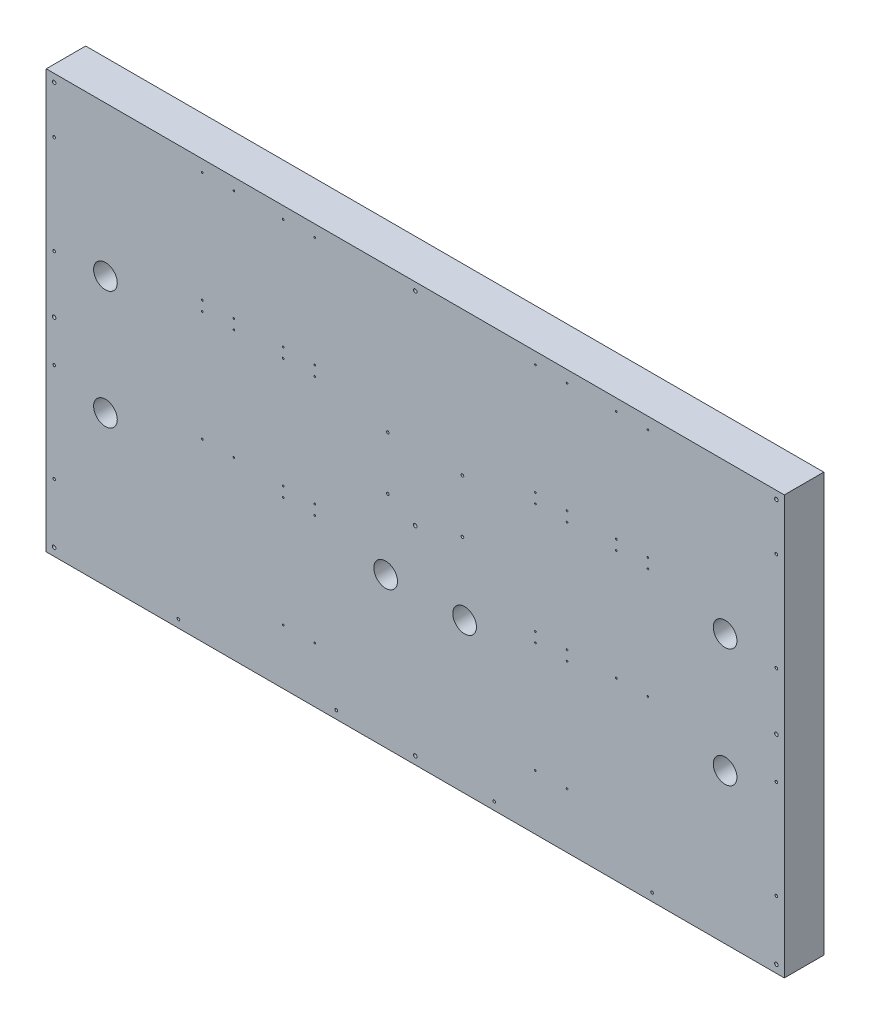
from build123d import *

# Parameters (mm, degrees)
SKETCH_1_W                           = 1870
SKETCH_1_H                           = 1060
EXTRUDE_1_DEPTH                      = 50
HOLE_WIZARD_M8_1_D                   = 6.8
PATTERN_LINEAR_1_COUNT               = 2
PATTERN_LINEAR_1_PITCH               = 135
PATTERN_LINEAR_1_COUNT_DIR2          = 2
PATTERN_LINEAR_1_PITCH_DIR2          = 189
HOLE_WIZARD_2_D                      = 9
HOLE_WIZARD_2_CBORE_D                = 15
HOLE_WIZARD_2_CBORE_DEPTH            = 50
PATTERN_LINEAR_2_COUNT               = 2
PATTERN_LINEAR_2_PITCH               = 515
PATTERN_LINEAR_3_COUNT               = 2
PATTERN_LINEAR_3_PITCH               = 915
PATTERN_LINEAR_3_COPY_1_D            = 9
PATTERN_LINEAR_3_COPY_1_CBORE_D      = 15
PATTERN_LINEAR_3_COPY_1_CBORE_DEPTH  = 50
HOLE_WIZARD_M5_1_D                   = 4.2
PATTERN_LINEAR_5_COUNT               = 2
PATTERN_LINEAR_5_PITCH               = 280
PATTERN_LINEAR_6_COUNT               = 2
PATTERN_LINEAR_6_PITCH               = 305
PATTERN_LINEAR_6_COPY_1_D            = 4.2
PATTERN_LINEAR_7_COUNT               = 2
PATTERN_LINEAR_7_PITCH               = 205
PATTERN_LINEAR_7_COPY_1_D            = 4.2
PATTERN_LINEAR_7_COPY_2_D            = 4.2
PATTERN_LINEAR_7_COPY_3_D            = 4.2
PATTERN_LINEAR_8_COUNT               = 2
PATTERN_LINEAR_8_PITCH               = 844
PATTERN_LINEAR_8_COPY_1_D            = 4.2
PATTERN_LINEAR_8_COPY_2_D            = 4.2
PATTERN_LINEAR_8_COPY_3_D            = 4.2
PATTERN_LINEAR_8_COPY_4_D            = 4.2
PATTERN_LINEAR_8_COPY_5_D            = 4.2
PATTERN_LINEAR_8_COPY_6_D            = 4.2
PATTERN_LINEAR_8_COPY_7_D            = 4.2
SKETCH_10_R                          = 2.1
CUT_EXTRUDE_1_DEPTH                  = 1080.409560825
PATTERN_LINEAR_9_COUNT               = 2
PATTERN_LINEAR_9_PITCH               = 639
SKETCH_12_R                          = 30
CUT_EXTRUDE_2_DEPTH                  = 1080.409560825
MIRROR_2_COPY_1_D                    = 9
MIRROR_2_COPY_1_CBORE_D              = 15
MIRROR_2_COPY_1_CBORE_DEPTH          = 50
SKETCH_13_R                          = 30
CUT_EXTRUDE_3_DEPTH                  = 1080.409560825
HOLE_WIZARD_M8_2_D                   = 6.8
PATTERN_LINEAR_10_COUNT              = 4
PATTERN_LINEAR_10_PITCH              = 250
MIRROR_3_COPY_1_D                    = 6.8
MIRROR_3_COPY_2_D                    = 6.8
MIRROR_3_COPY_3_D                    = 6.8
HOLE_WIZARD_M8_3_D                   = 6.8
PATTERN_LINEAR_11_COUNT              = 4
PATTERN_LINEAR_11_PITCH              = 400
PATTERN_LINEAR_12_COUNT              = 2
PATTERN_LINEAR_12_PITCH              = 1020
PATTERN_LINEAR_13_COPY_1_D           = 9
PATTERN_LINEAR_13_COPY_1_CBORE_D     = 15
PATTERN_LINEAR_13_COPY_1_CBORE_DEPTH = 50
PATTERN_LINEAR_13_COPY_2_D           = 9
PATTERN_LINEAR_13_COPY_2_CBORE_D     = 15
PATTERN_LINEAR_13_COPY_2_CBORE_DEPTH = 50
MIRROR_4_COPY_1_D                    = 9
MIRROR_4_COPY_1_CBORE_D              = 15
MIRROR_4_COPY_1_CBORE_DEPTH          = 50
MIRROR_4_COPY_2_D                    = 9
MIRROR_4_COPY_2_CBORE_D              = 15
MIRROR_4_COPY_2_CBORE_DEPTH          = 50


with BuildPart() as part:
    # 草图1 → 凸台-拉伸1 (new, symmetric)
    with BuildSketch(Plane.XY):
        Rectangle(SKETCH_1_W, SKETCH_1_H)
    extrude(amount=EXTRUDE_1_DEPTH, both=True)

    # M8 螺纹孔1 (through all)
    with Locations(Plane.XY.offset(50)):
        with Locations((-69.5, 30)):
            hole_wizard_m8_1 = Hole(HOLE_WIZARD_M8_1_D / 2)

    # 阵列(线性)1: Hole Wizard M8 _1 2 × 2
    with Locations(*[(j * PATTERN_LINEAR_1_PITCH_DIR2, i * PATTERN_LINEAR_1_PITCH, 0) for i in range(PATTERN_LINEAR_1_COUNT) for j in range(PATTERN_LINEAR_1_COUNT_DIR2) if (i, j) != (0, 0)]):
        add(hole_wizard_m8_1, mode=Mode.SUBTRACT)

    # 打孔尺寸(%根据)内六角圆柱头螺钉的类型2 (through all)
    with Locations(Plane(origin=(0, 0, -50), x_dir=(-1, 0, 0), z_dir=(0, 0, -1))):
        with Locations((-915, 510)):
            hole_wizard_2 = CounterBoreHole(HOLE_WIZARD_2_D / 2, HOLE_WIZARD_2_CBORE_D / 2, HOLE_WIZARD_2_CBORE_DEPTH)

    # 阵列(线性)2: 打孔尺寸(%根据)内六角圆柱头螺钉的类型2 ×2
    with Locations(*[(0, -i * PATTERN_LINEAR_2_PITCH, 0) for i in range(1, PATTERN_LINEAR_2_COUNT)]):
        add(hole_wizard_2, mode=Mode.SUBTRACT)

    # 阵列(线性)3: 打孔尺寸(%根据)内六角圆柱头螺钉的类型2 ×2
    with Locations(*[(-i * PATTERN_LINEAR_3_PITCH, 0, 0) for i in range(1, PATTERN_LINEAR_3_COUNT)]):
        add(hole_wizard_2, mode=Mode.SUBTRACT)

    # 阵列(线性)3 copy 1 (through all)
    with Locations(Plane(origin=(-915, -515, -50), x_dir=(-1, 0, 0), z_dir=(0, 0, -1))):
        with Locations((-915, 510)):
            CounterBoreHole(PATTERN_LINEAR_3_COPY_1_D / 2, PATTERN_LINEAR_3_COPY_1_CBORE_D / 2, PATTERN_LINEAR_3_COPY_1_CBORE_DEPTH)

    # M5 螺纹孔1 (through all)
    with Locations(Plane(origin=(0, 0, -50), x_dir=(-1, 0, 0), z_dir=(0, 0, -1))):
        with Locations((-589.5, 500), (-509.5, 500)):
            hole_wizard_m5_1 = Hole(HOLE_WIZARD_M5_1_D / 2)

    # 阵列(线性)5: M5 螺纹孔1 ×2
    with Locations(*[(0, -i * PATTERN_LINEAR_5_PITCH, 0) for i in range(1, PATTERN_LINEAR_5_COUNT)]):
        add(hole_wizard_m5_1, mode=Mode.SUBTRACT)

    # 阵列(线性)6: M5 螺纹孔1 ×2
    with Locations(*[(0, -i * PATTERN_LINEAR_6_PITCH, 0) for i in range(1, PATTERN_LINEAR_6_COUNT)]):
        add(hole_wizard_m5_1, mode=Mode.SUBTRACT)

    # 阵列(线性)6 copy 1 (through all)
    with Locations(Plane(origin=(0, -585, -50), x_dir=(-1, 0, 0), z_dir=(0, 0, -1))):
        with Locations((-589.5, 500), (-509.5, 500)):
            Hole(PATTERN_LINEAR_6_COPY_1_D / 2)

    # 阵列(线性)7: M5 螺纹孔1 ×2
    with Locations(*[(-i * PATTERN_LINEAR_7_PITCH, 0, 0) for i in range(1, PATTERN_LINEAR_7_COUNT)]):
        add(hole_wizard_m5_1, mode=Mode.SUBTRACT)

    # 阵列(线性)7 copy 1 (through all)
    with Locations(Plane(origin=(-205, -280, -50), x_dir=(-1, 0, 0), z_dir=(0, 0, -1))):
        with Locations((-589.5, 500), (-509.5, 500)):
            Hole(PATTERN_LINEAR_7_COPY_1_D / 2)

    # 阵列(线性)7 copy 2 (through all)
    with Locations(Plane(origin=(-205, -305, -50), x_dir=(-1, 0, 0), z_dir=(0, 0, -1))):
        with Locations((-589.5, 500), (-509.5, 500)):
            Hole(PATTERN_LINEAR_7_COPY_2_D / 2)

    # 阵列(线性)7 copy 3 (through all)
    with Locations(Plane(origin=(-205, -585, -50), x_dir=(-1, 0, 0), z_dir=(0, 0, -1))):
        with Locations((-589.5, 500), (-509.5, 500)):
            Hole(PATTERN_LINEAR_7_COPY_3_D / 2)

    # 阵列(线性)8: M5 螺纹孔1 ×2
    with Locations(*[(-i * PATTERN_LINEAR_8_PITCH, 0, 0) for i in range(1, PATTERN_LINEAR_8_COUNT)]):
        add(hole_wizard_m5_1, mode=Mode.SUBTRACT)

    # 阵列(线性)8 copy 1 (through all)
    with Locations(Plane(origin=(-844, -280, -50), x_dir=(-1, 0, 0), z_dir=(0, 0, -1))):
        with Locations((-589.5, 500), (-509.5, 500)):
            Hole(PATTERN_LINEAR_8_COPY_1_D / 2)

    # 阵列(线性)8 copy 2 (through all)
    with Locations(Plane(origin=(-844, -305, -50), x_dir=(-1, 0, 0), z_dir=(0, 0, -1))):
        with Locations((-589.5, 500), (-509.5, 500)):
            Hole(PATTERN_LINEAR_8_COPY_2_D / 2)

    # 阵列(线性)8 copy 3 (through all)
    with Locations(Plane(origin=(-844, -585, -50), x_dir=(-1, 0, 0), z_dir=(0, 0, -1))):
        with Locations((-589.5, 500), (-509.5, 500)):
            Hole(PATTERN_LINEAR_8_COPY_3_D / 2)

    # 阵列(线性)8 copy 4 (through all)
    with Locations(Plane(origin=(-1049, 0, -50), x_dir=(-1, 0, 0), z_dir=(0, 0, -1))):
        with Locations((-589.5, 500), (-509.5, 500)):
            Hole(PATTERN_LINEAR_8_COPY_4_D / 2)

    # 阵列(线性)8 copy 5 (through all)
    with Locations(Plane(origin=(-1049, -280, -50), x_dir=(-1, 0, 0), z_dir=(0, 0, -1))):
        with Locations((-589.5, 500), (-509.5, 500)):
            Hole(PATTERN_LINEAR_8_COPY_5_D / 2)

    # 阵列(线性)8 copy 6 (through all)
    with Locations(Plane(origin=(-1049, -305, -50), x_dir=(-1, 0, 0), z_dir=(0, 0, -1))):
        with Locations((-589.5, 500), (-509.5, 500)):
            Hole(PATTERN_LINEAR_8_COPY_6_D / 2)

    # 阵列(线性)8 copy 7 (through all)
    with Locations(Plane(origin=(-1049, -585, -50), x_dir=(-1, 0, 0), z_dir=(0, 0, -1))):
        with Locations((-589.5, 500), (-509.5, 500)):
            Hole(PATTERN_LINEAR_8_COPY_7_D / 2)

    # 草图10 → 切除-拉伸1 (cut, through all)
    with BuildSketch(Plane(origin=(0, 0, -50), x_dir=(-1, 0, 0), z_dir=(0, 0, -1))):
        with Locations((-304.5, -390)):
            Circle(SKETCH_10_R)
        with Locations((-384.5, -390)):
            Circle(SKETCH_10_R)
        with Locations((-304.5, -110)):
            Circle(SKETCH_10_R)
        with Locations((-384.5, -110)):
            Circle(SKETCH_10_R)
    cut_extrude_1 = extrude(amount=-CUT_EXTRUDE_1_DEPTH, mode=Mode.SUBTRACT)

    # 阵列(线性)9: 切除-拉伸1 ×2
    with Locations(*[(-i * PATTERN_LINEAR_9_PITCH, 0, 0) for i in range(1, PATTERN_LINEAR_9_COUNT)]):
        add(cut_extrude_1, mode=Mode.SUBTRACT)

    # 草图12 → 切除-拉伸2 (cut, through all)
    with BuildSketch(Plane(origin=(0, 0, -50), x_dir=(-1, 0, 0), z_dir=(0, 0, -1))):
        with Locations((-785, 150)):
            Circle(SKETCH_12_R)
        with Locations((-785, -150)):
            Circle(SKETCH_12_R)
    cut_extrude_2 = extrude(amount=-CUT_EXTRUDE_2_DEPTH, mode=Mode.SUBTRACT)

    # 镜向1: 切除-拉伸2 across plane
    add(cut_extrude_2.mirror(Plane(origin=(0, 0, 0), x_dir=(0, 0, 1), z_dir=(1, 0, 0))), mode=Mode.SUBTRACT)

    # 镜向2: 打孔尺寸(%根据)内六角圆柱头螺钉的类型2 across plane
    add(hole_wizard_2.mirror(Plane(origin=(0, 0, 0), x_dir=(0, 0, 1), z_dir=(1, 0, 0))), mode=Mode.SUBTRACT)

    # 镜向2 copy 1 (through all)
    with Locations(Plane(origin=(0, -515, -50), x_dir=(1, 0, 0), z_dir=(0, 0, -1))):
        with Locations((-915, -510)):
            CounterBoreHole(MIRROR_2_COPY_1_D / 2, MIRROR_2_COPY_1_CBORE_D / 2, MIRROR_2_COPY_1_CBORE_DEPTH)

    # 草图13 → 切除-拉伸3 (cut, through all)
    with BuildSketch(Plane(origin=(0, 0, -50), x_dir=(-1, 0, 0), z_dir=(0, 0, -1))):
        with Locations((-125, -150)):
            Circle(SKETCH_13_R)
        with Locations((75, -150)):
            Circle(SKETCH_13_R)
    extrude(amount=-CUT_EXTRUDE_3_DEPTH, mode=Mode.SUBTRACT)

    # M8 螺纹孔2 (through all)
    with Locations(Plane(origin=(0, 0, -50), x_dir=(-1, 0, 0), z_dir=(0, 0, -1))):
        with Locations((-915, 390)):
            hole_wizard_m8_2 = Hole(HOLE_WIZARD_M8_2_D / 2)

    # 阵列(线性)10: M8 螺纹孔2 ×4
    with Locations(*[(0, -i * PATTERN_LINEAR_10_PITCH, 0) for i in range(1, PATTERN_LINEAR_10_COUNT)]):
        add(hole_wizard_m8_2, mode=Mode.SUBTRACT)

    # 镜向3: M8 螺纹孔2 across plane
    add(hole_wizard_m8_2.mirror(Plane(origin=(0, 0, 0), x_dir=(0, 0, 1), z_dir=(1, 0, 0))), mode=Mode.SUBTRACT)

    # 镜向3 copy 1 (through all)
    with Locations(Plane(origin=(0, -250, -50), x_dir=(1, 0, 0), z_dir=(0, 0, -1))):
        with Locations((-915, -390)):
            Hole(MIRROR_3_COPY_1_D / 2)

    # 镜向3 copy 2 (through all)
    with Locations(Plane(origin=(0, -500, -50), x_dir=(1, 0, 0), z_dir=(0, 0, -1))):
        with Locations((-915, -390)):
            Hole(MIRROR_3_COPY_2_D / 2)

    # 镜向3 copy 3 (through all)
    with Locations(Plane(origin=(0, -750, -50), x_dir=(1, 0, 0), z_dir=(0, 0, -1))):
        with Locations((-915, -390)):
            Hole(MIRROR_3_COPY_3_D / 2)

    # M8 螺纹孔3 (through all)
    with Locations(Plane(origin=(0, 0, -50), x_dir=(-1, 0, 0), z_dir=(0, 0, -1))):
        with Locations((-600, -510)):
            hole_wizard_m8_3 = Hole(HOLE_WIZARD_M8_3_D / 2)

    # 阵列(线性)11: M8 螺纹孔3 ×4
    with Locations(*[(-i * PATTERN_LINEAR_11_PITCH, 0, 0) for i in range(1, PATTERN_LINEAR_11_COUNT)]):
        add(hole_wizard_m8_3, mode=Mode.SUBTRACT)

    # 阵列(线性)12: 打孔尺寸(%根据)内六角圆柱头螺钉的类型2 ×2
    with Locations(*[(0, -i * PATTERN_LINEAR_12_PITCH, 0) for i in range(1, PATTERN_LINEAR_12_COUNT)]):
        add(hole_wizard_2, mode=Mode.SUBTRACT)

    # 阵列(线性)13 copy 1 (through all)
    with Locations(Plane(origin=(-915, -1020, -50), x_dir=(-1, 0, 0), z_dir=(0, 0, -1))):
        with Locations((-915, 510)):
            CounterBoreHole(PATTERN_LINEAR_13_COPY_1_D / 2, PATTERN_LINEAR_13_COPY_1_CBORE_D / 2, PATTERN_LINEAR_13_COPY_1_CBORE_DEPTH)

    # 阵列(线性)13 copy 2 (through all)
    with Locations(Plane(origin=(-915, 0, -50), x_dir=(-1, 0, 0), z_dir=(0, 0, -1))):
        with Locations((-915, 510)):
            CounterBoreHole(PATTERN_LINEAR_13_COPY_2_D / 2, PATTERN_LINEAR_13_COPY_2_CBORE_D / 2, PATTERN_LINEAR_13_COPY_2_CBORE_DEPTH)

    # 镜向4 copy 1 (through all)
    with Locations(Plane(origin=(0, -1020, -50), x_dir=(1, 0, 0), z_dir=(0, 0, -1))):
        with Locations((-915, -510)):
            CounterBoreHole(MIRROR_4_COPY_1_D / 2, MIRROR_4_COPY_1_CBORE_D / 2, MIRROR_4_COPY_1_CBORE_DEPTH)

    # 镜向4 copy 2 (through all)
    with Locations(Plane(origin=(0, 0, -50), x_dir=(1, 0, 0), z_dir=(0, 0, -1))):
        with Locations((-915, -510)):
            CounterBoreHole(MIRROR_4_COPY_2_D / 2, MIRROR_4_COPY_2_CBORE_D / 2, MIRROR_4_COPY_2_CBORE_DEPTH)


solid = part.part
